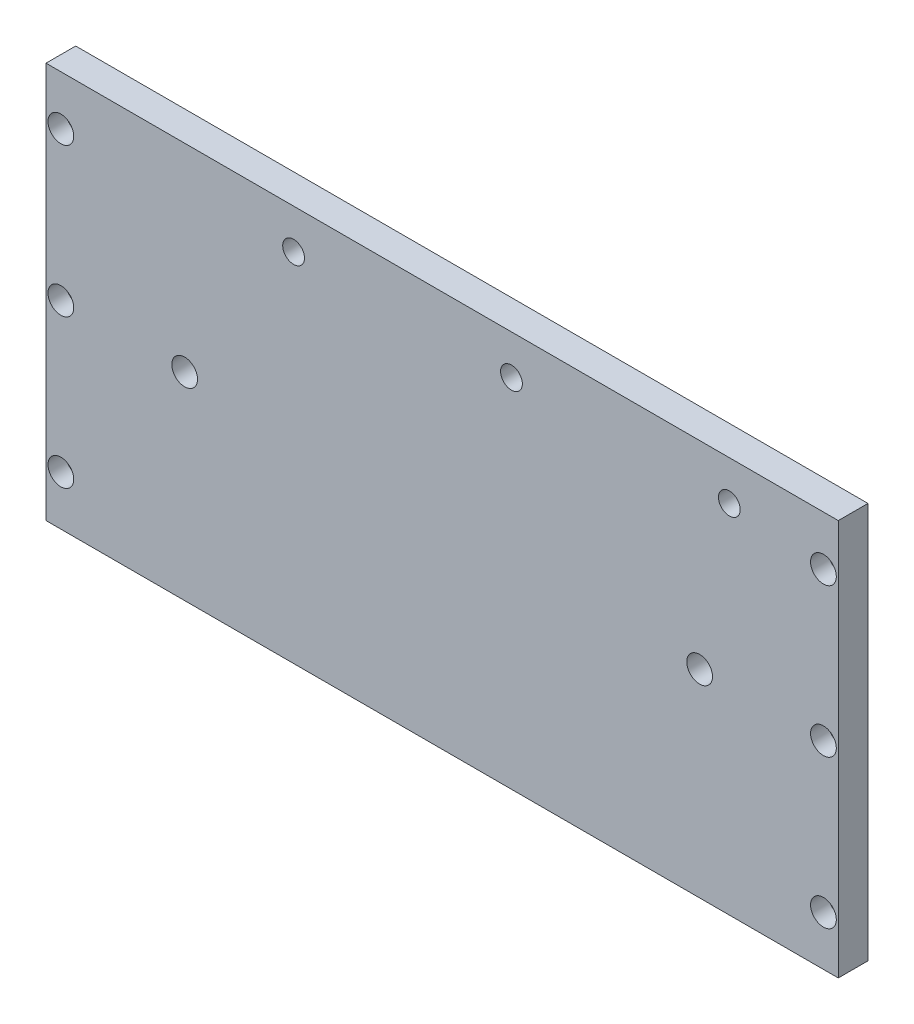
SolidWorks part; units mm, degrees
ref_plane "Front Plane" through (0, 0, 0) normal (0, 0, 1) x (1, 0, 0)
ref_plane "Top Plane" through (0, 0, 0) normal (0, 1, 0) x (1, 0, 0)
ref_plane "Right Plane" through (0, 0, 0) normal (1, 0, 0) x (0, 0, -1)
sketch "Sketch1" plane through (0, 0, 0) normal (0, 0, 1) x (1, 0, 0)
  line L1 (200, -100) -> (-200, -100)
  line L2 (200, -100) -> (200, 100)
  line L3 (200, 100) -> (-200, 100)
  line L4 (-200, -100) -> (-200, 100)
  line L5 (200, -100) -> (-200, 100) construction
  line L6 (200, 100) -> (-200, -100) construction
  point P1 (0, 0)
  dimension "D1" = 400
  dimension "D2" = 200
extrude "Boss-Extrude1" add sketch "Sketch1" along normal blind 15
sketch "Sketch2" plane through (0, 0, 15) normal (0, 0, 1) x (1, 0, 0)
  circle A0 centre (-192.5, 75) radius 6.5
  dimension "D1" = 13
extrude "Cut-Extrude1" cut sketch "Sketch2" against normal blind 9
pattern_linear "LPattern1" count 3 spacing 75 along (0, -1, 0) of "Cut-Extrude1"
mirror "Mirror1" about plane through (0, 0, 0) normal (1, 0, 0) of "LPattern1", "Cut-Extrude1"
sketch "Sketch3" plane through (0, 0, 15) normal (0, 0, 1) x (1, 0, 0)
  circle A0 centre (-192.5, 75) radius 4.5
  dimension "D1" = 9
extrude "Cut-Extrude2" cut sketch "Sketch3" against normal blind 85
pattern_linear "LPattern2" count 3 spacing 75 along (0, -1, 0) of "Cut-Extrude2"
mirror "Mirror2" about plane through (0, 0, 0) normal (1, 0, 0) of "LPattern2", "Cut-Extrude2"
sketch "Sketch4" plane through (0, 0, 15) normal (0, 0, 1) x (1, 0, 0)
  line L0 (8.25, 0) -> (-8.25, 0) construction
  line L1 (0, -8.25) -> (0, 8.25) construction
  circle A0 centre (-130, 0) radius 6.5
  dimension "D1" = 13
  dimension "D2" = 130
extrude "Cut-Extrude3" cut sketch "Sketch4" against normal blind 85
pattern_linear "LPattern3" count 3 spacing 130 along (1, 0, 0) skipping (1, 0) of "Cut-Extrude3"
sketch "Sketch5" plane through (0, 0, 15) normal (0, 0, 1) x (1, 0, 0)
  line L0 (200, 100) -> (-200, 100) construction
  line L1 (0, -8.25) -> (0, 8.25) construction
  circle A0 centre (-75, 80) radius 5.5
  dimension "D1" = 11
  dimension "D2" = 20
  dimension "D3" = 75
extrude "Cut-Extrude4" cut sketch "Sketch5" against normal blind 51
pattern_linear "LPattern4" count 3 spacing 110 along (1, 0, 0) of "Cut-Extrude4"
